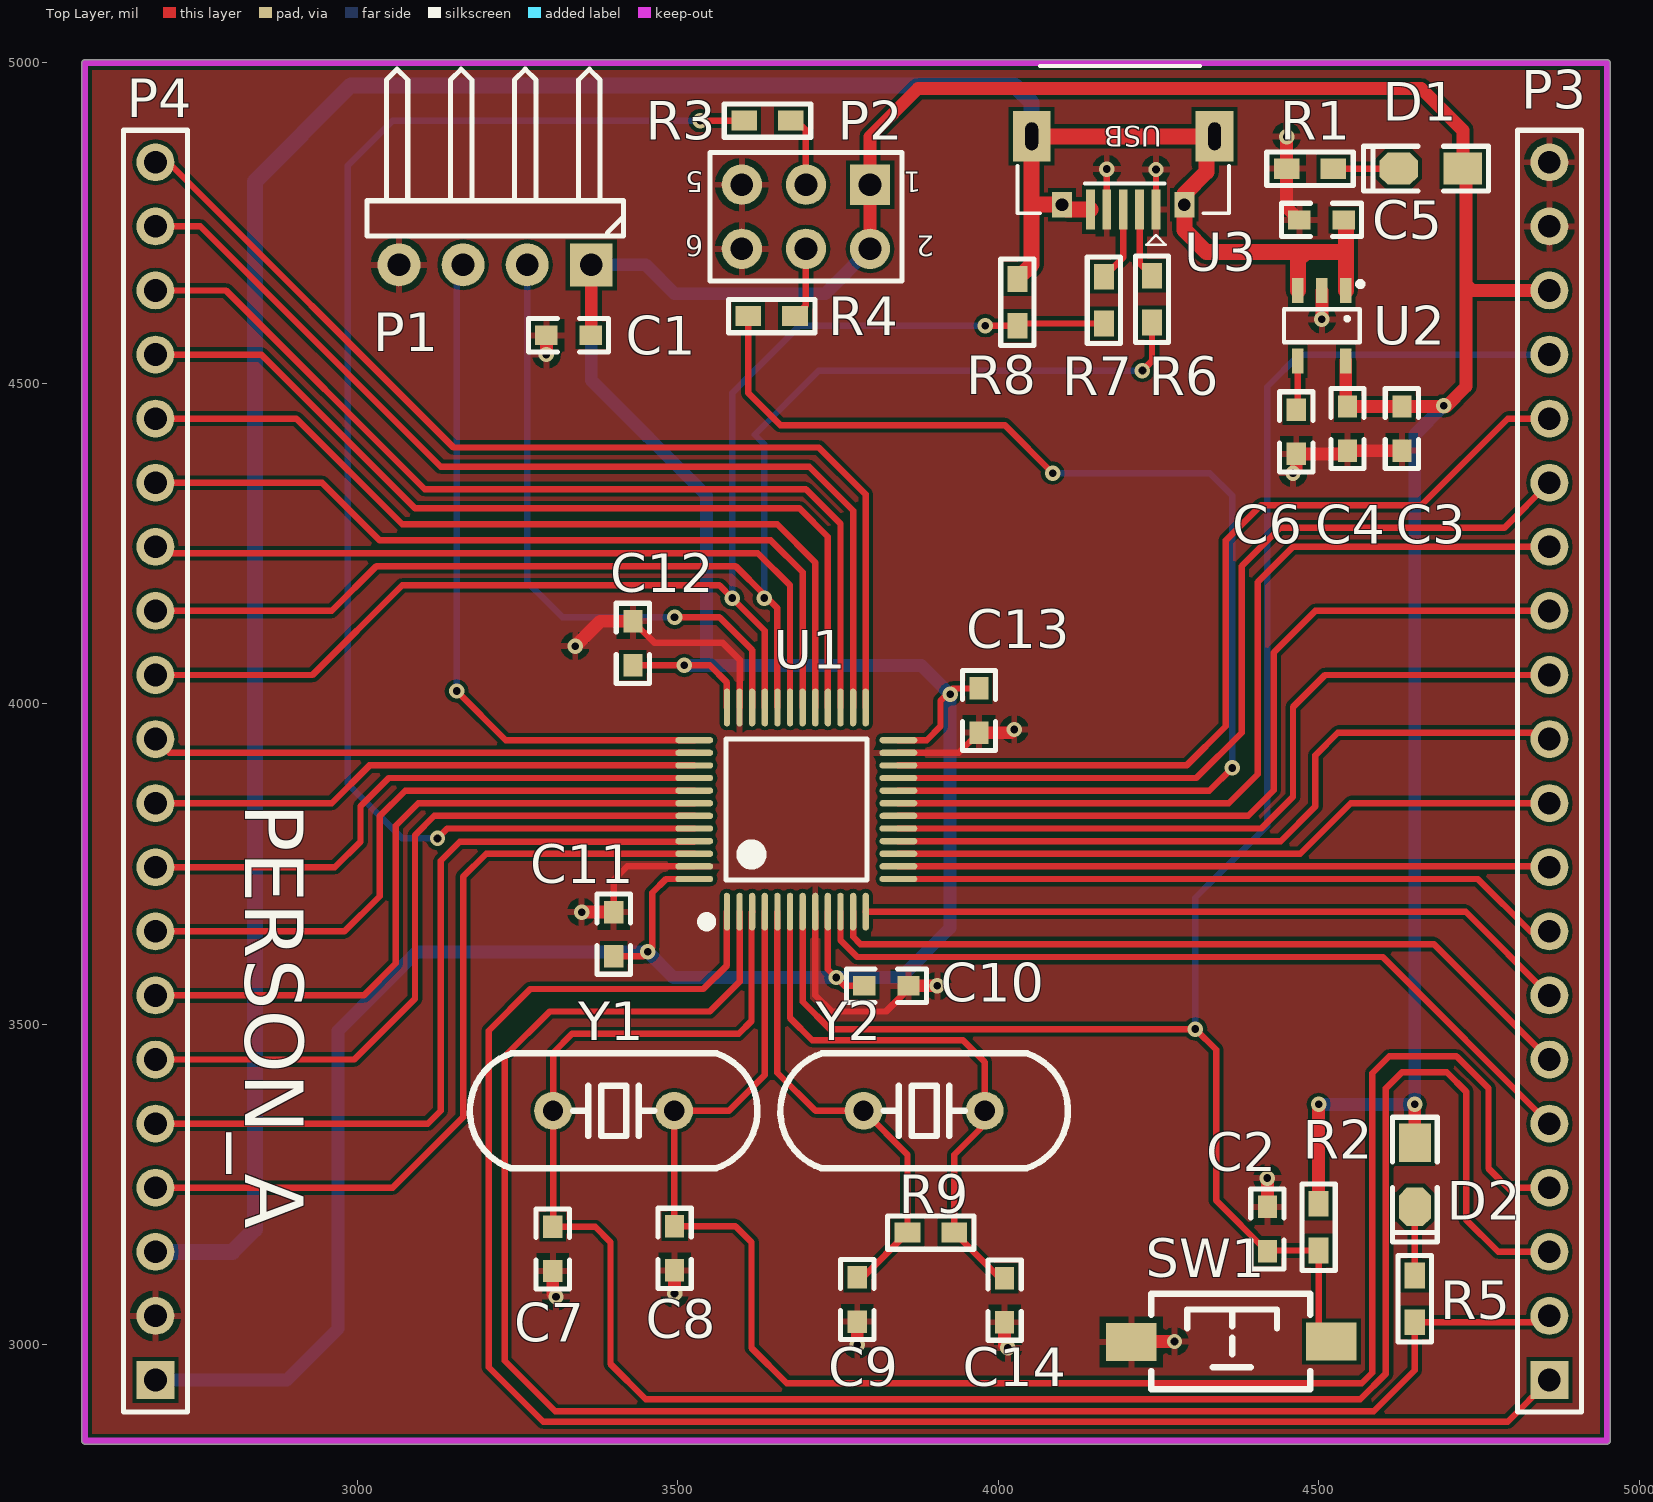
[diagram p0: Top Layer view]
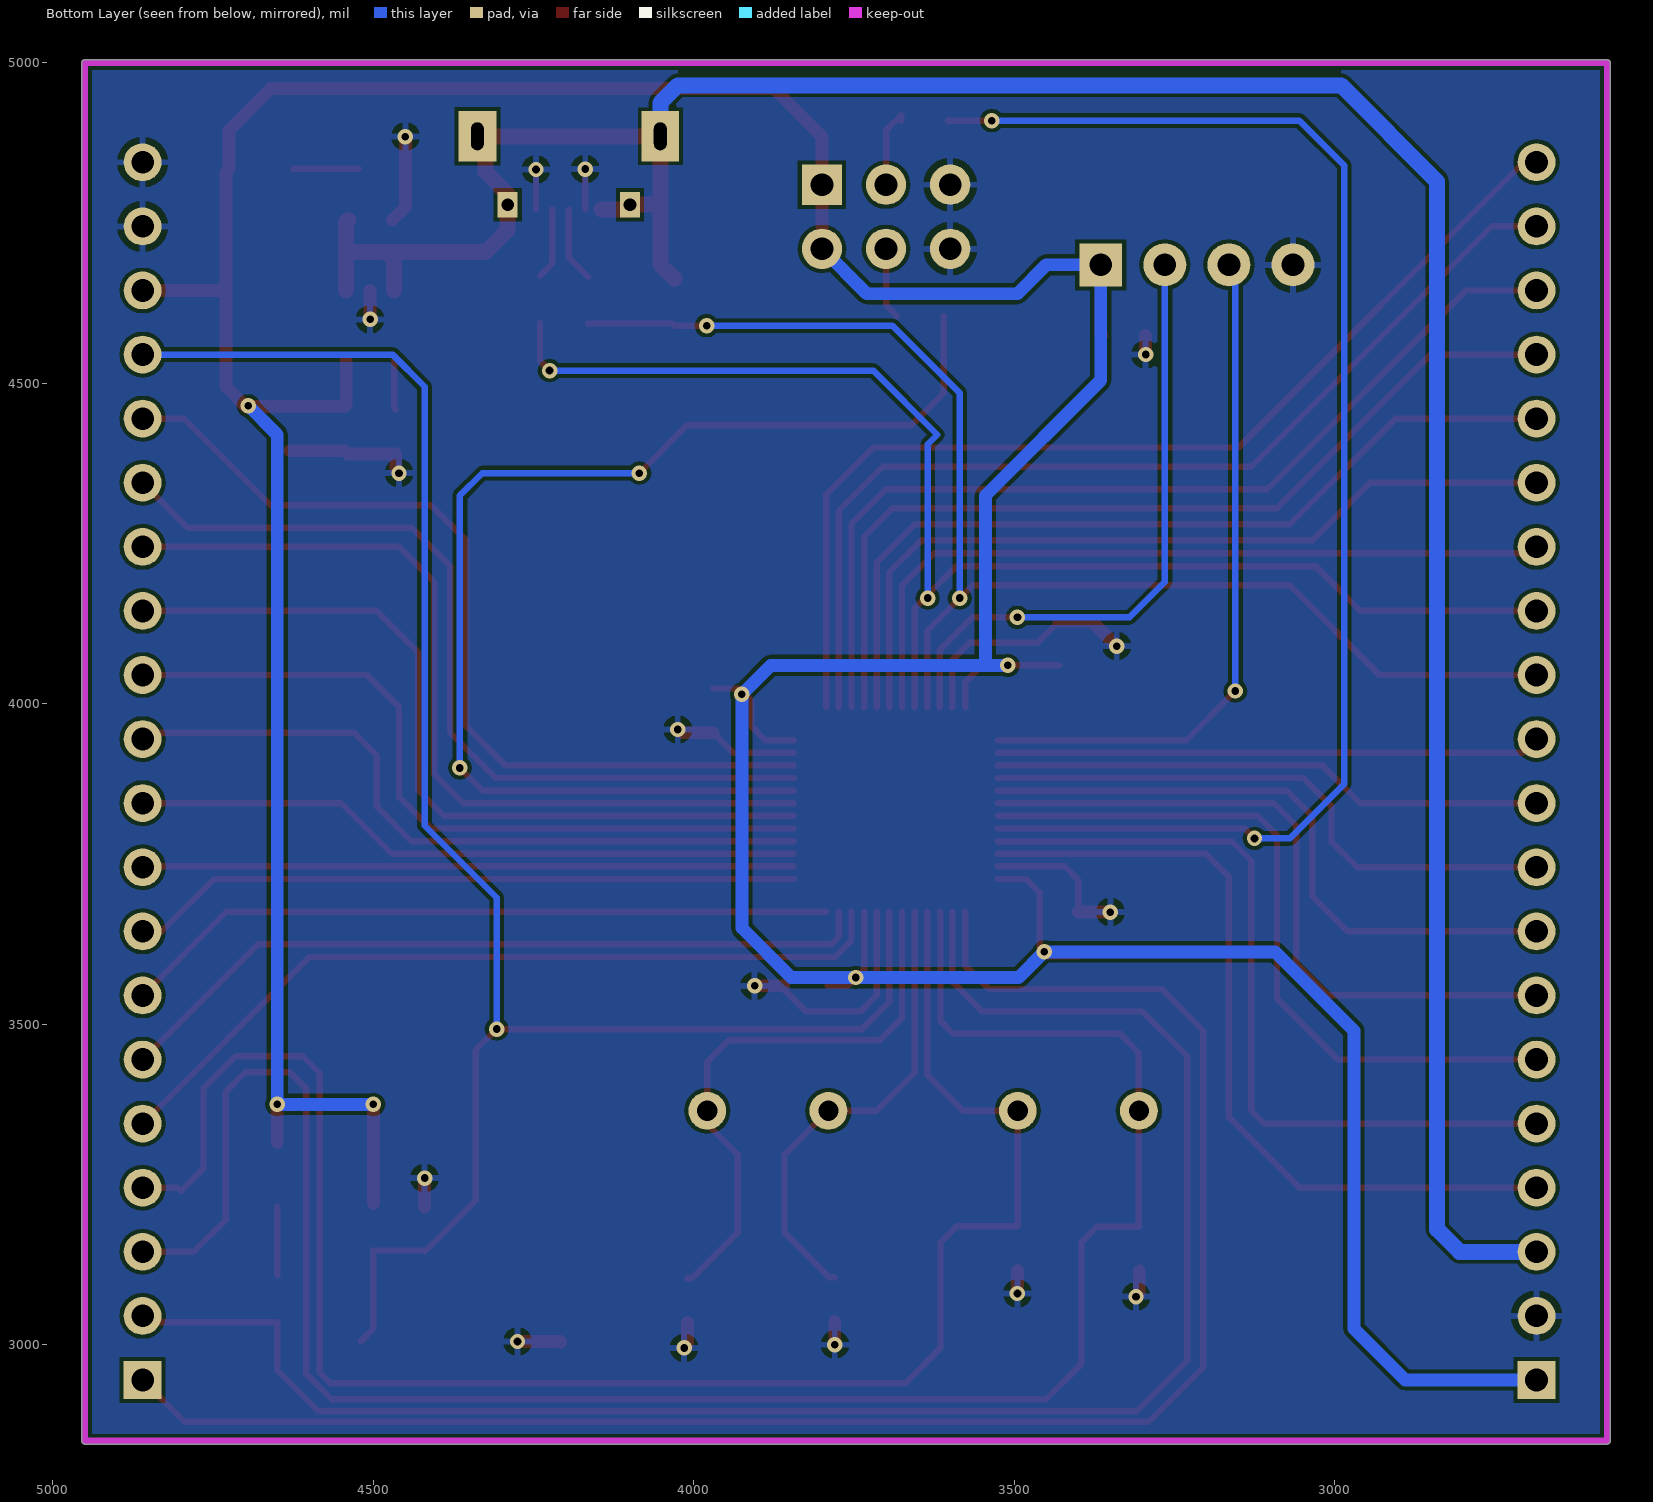
[diagram p1: Bottom Layer view, seen from below]
# Altium PCB MISC82227.PcbDoc
Units mil, origin at the board's own origin, x right, y up, seen from the top; angles counter-clockwise.
Board outline 2385.03 x 2160.03 mil, 2 copper layers (Top Layer, Bottom Layer); 35 components, 50 nets, 168 pads, 34 vias.

## Layer stack, top to bottom (the 12.6 mil dielectric is the usual default, probably not edited)
Top Solder: solder mask 0.4, Solder Resist, Dk 3.5
Top Layer: signal copper 1.4
Dielectric 1: dielectric 12.6, FR-4, Dk 4.8
Bottom Layer: signal copper 1.4
Bottom Solder: solder mask 0.4, Solder Resist, Dk 3.5

## Board outline
2575,2844.99 cw(c2575,2850) 2569.99,2850 2569.99,5000 cw(c2575,5000) 2575,5005.02 4950,5005.02 cw(c4950,5000) 4955.02,5000 4955.02,2850 cw(c4950,2850) 4950,2844.99

## Design rules (kind name [scope] priority, off if disabled: settings)
Clearance [All] p1: gap=6
MinimumSolderMaskSliver [All] p1: minsoldermaskwidth=0
PolygonConnect [All] p1: connectstyle=Relief reliefconductorwidth=10 reliefentries=4 polygonreliefangle="90 Angle" airgapwidth=10
RoutingVias [All] p1: holewidth=28 width=50 viastyle="Through Hole" minholewidth=28 minwidth=50 maxholewidth=28 maxwidth=50
SilkToSilkClearance [All] p1: silktosilkclearance=0
SilkToSolderMaskClearance [IsPad] p1: minsilkscreentomaskgap=0 clearancetoexposedcopper=TRUE
SolderMaskExpansion [All] p1: expansion=4
Width [All] p1: maxlimit=30 minlimit=10 preferedwidth=10
27 further rules are at their usual default settings.

## Components (designator, comment, footprint, x,y, rotation, side; value= is the part's Value field where it differs from the comment)
C1 "105 C0603" "C 0603" 3330,4575 r0 top
C2 "105 C0603" "C 0603" 4420,3180 r270 top
C3 "105 C0603" "C 0603" 4630,4430 r90 top
C4 "105 C0603" "C 0603" 4545,4430 r90 top
C5 "105 C0603" "C 0603" 4505,4755 r0 top
C6 "105 C0603" "C 0603" 4465,4425 r90 top
C7 "22P,0603" "C 0603" 3305,3149 r270 top
C8 "22P,0603" "C 0603" 3495,3150 r270 top
C9 "22P,0603" "C 0603" 3780,3070 r270 top
C10 "105 C0603" "C 0603" 3825,3560 r180 top
C11 "105 C0603" "C 0603" 3400,3640 r270 top
C12 "105 C0603" "C 0603" 3430,4094 r270 top
C13 "105 C0603" "C 0603" 3970,3990 r90 top
C14 "22P,0603" "C 0603" 4010,3069 r270 top
D1 "LED" "LED 0805G" 4675,4835 r180 top
D2 "LED" "LED 0805G" 4650,3265 r270 top
P1 "SWD" HDR-1X4_H 3365,4685 r180 top
P2 "Header 3X2" HDR-3X2 3800,4810 r180 top
P3 "Header 20" HDR1X20 4860,2945 r90 top
P4 "Header 20" HDR1X20 2685,2945 r90 top
R1 "10K R0603" "R 0603" 4486.5,4835 r180 top
R2 "10K R0603" "R 0603" 4500,3183.5 r90 top
R3 "10K R0603" "R 0603" 3640,4910 r0 top
R4 "10K R0603" "R 0603" 3646.5,4605 r180 top
R5 "10K R0603" "R 0603" 4650,3071.5 r270 top
R6 "20R,0603" "R 0603" 4240,4631.5 r270 top
R7 "20R0603" "R 0603" 4165,4630 r270 top
R8 "4.7K,0603" "R 0603" 4030,4626.5 r270 top
R9 "1M0603" "R 0603" 3895,3175 r180 top
SW1 "SW-PB_V" "TSW SMD-3*6*2.5" 4365,3005 r0 top
U1 "stm32f103c8t6_48pin" "TQFP48 7x7_L" 3685,3835 r0 top
U2 "RT9193" SOT23-5L 4505,4590 r180 top
U3 "USB-mrico" USB-micro_B 4195,4885.51 r180 top
Y1 "32.768K" "XTAL-49S DIP" 3400,3365 r180 top
Y2 "8M" "XTAL-49S DIP" 3884.49,3365 r180 top

## Footprints (in the part's own frame and the unit in brackets; to place one, negate y for a bottom-side part, rotate by r counter-clockwise, add the part's x,y. Pads: shape width x height; smd on the part's side, far side on the other; paste and mask are expansions set on the pad)
"C 0603" [mil] "无极性贴片电容"
  rect 35x30 smd: 1(-35,0) 2(34,0)
  silkscreen extent -63,-26 62,26, body extent -31,-16 31,16, height 32
HDR1X20 [mm] "Connector; Header; 20 Position"
  rect 1.5x1.5 hole 0.9: 1(0,0)
  round 1.5 hole 0.9: 2(2.54,0) 3(5.08,0) 4(7.62,0) 5(10.16,0) 6(12.7,0) 7(15.24,0) 8(17.78,0) 9(20.32,0) 10(22.86,0) 11(25.4,0) 12(27.94,0) 13(30.48,0) 14(33.02,0) 15(35.56,0) 16(38.1,0) 17(40.64,0) 18(43.18,0) 19(45.72,0) 20(48.26,0)
  silkscreen extent -1.27,-1.27 49.53,1.27
HDR-1X4_H [mm] "弯脚排针，4脚"
  rect 1.7x1.7 hole 0.9: 1(0,0)
  round 1.7 hole 0.9: 2(2.54,0) 3(5.08,0) 4(7.62,0)
  silkscreen extent -1.27,-7.76 8.89,-1.14, body extent -1.27,-7.77 8.89,1.27, height 4.85
HDR-3X2 [mm] "双排排针，3x2脚"
  rect 1.6x1.6 hole 0.9: 1(0,0)
  round 1.6 hole 0.9: 2(0,2.54) 3(2.54,0) 4(2.54,2.54) 5(5.08,0) 6(5.08,2.54)
  silkscreen extent -1.27,-1.27 6.35,3.81, body extent -1.27,-1.27 6.35,3.81, height 8.5
"LED 0805G" [mil] "绿色0805LED"
  rect 60x50 smd: 1(-50,0)
  oct 60x50 smd: 2(50,0)
  silkscreen extent -90,-35 105,35, body extent -39,-25 39,25, height 32
"R 0603" [mil] "1/10W贴片电阻"
  rect 40x31.5 smd: 1(-36.5,0) 2(36.5,0)
  silkscreen extent -68,-26 68,26, body extent -31,-16 31,16, height 16
SOT23-5L [mm] "3x1.6x1.1mm(长宽高)"
  rect 0.45x1 smd: 1(-0.95,-1.4) 2(0,-1.4) 3(0.95,-1.4) 4(0.95,1.4) 5(-0.95,1.4)
  silkscreen extent -1.6,-1.73 1.5,0.66, body extent -1.5,-1.4 1.5,1.4, height 1.15
"TQFP48 7x7_L" [mm] "48脚，体宽：7x7mm, 脚距：0.5mm"
  oval 0.25x1.5 smd: 1(-2.75,-4.046) 2(-2.25,-4.046) 3(-1.75,-4.046) 4(-1.25,-4.046) 5(-0.75,-4.046) 6(-0.25,-4.046) 7(0.25,-4.046) 8(0.75,-4.046) 9(1.25,-4.046) 10(1.75,-4.046) 11(2.25,-4.046) 12(2.75,-4.046) 25(2.75,4.046) 26(2.25,4.046) 27(1.75,4.046) 28(1.25,4.046) 29(0.75,4.046) 30(0.25,4.046) 31(-0.25,4.046) 32(-0.75,4.046) 33(-1.25,4.046) 34(-1.75,4.046) 35(-2.25,4.046) 36(-2.75,4.046)
  oval 1.5x0.25 smd: 13(4.046,-2.75) 14(4.046,-2.25) 15(4.046,-1.75) 16(4.046,-1.25) 17(4.046,-0.75) 18(4.046,-0.25) 19(4.046,0.25) 20(4.046,0.75) 21(4.046,1.25) 22(4.046,1.75) 23(4.046,2.25) 24(4.046,2.75) 37(-4.046,2.75) 38(-4.046,2.25) 39(-4.046,1.75) 40(-4.046,1.25) 41(-4.046,0.75) 42(-4.046,0.25) 43(-4.046,-0.25) 44(-4.046,-0.75) 45(-4.046,-1.25) 46(-4.046,-1.75) 47(-4.046,-2.25) 48(-4.046,-2.75)
  silkscreen extent -3.68,-4.57 2.79,2.79, body extent -4.5,-4.5 4.5,4.5, height 1.05
"TSW SMD-3*6*2.5" [mm] "3*6*2.5mm"
  rect 2x1.5 smd: 1(-3.996,-0.02) 2(3.937,0)
  silkscreen extent -3.21,-1.9 3.09,1.9, body extent -4,-1.88 4,1.62, height 2.59
USB-micro_B [mm] "micro型USB ，5.7*7.8*2.5mm"
  rect 0.35x1.6 smd: 1(-1.3,2.9) 2(-0.65,2.9) 3(0,2.9) 4(0.65,2.9) 5(1.3,2.9)
  rect 1.5x2 hole 0.5 slot 1.1 at 90 deg: 5(-3.625,0) 5(3.625,0)
  rect 0.8x1 hole 0.5: 5(-2.425,2.71) 5(2.425,2.71)
  silkscreen extent -4.19,-2.79 4.19,4.3, body extent -4,-2.71 4,2.89, height 2.8
"XTAL-49S DIP" [mm]
  round 1.5 hole 0.8: 1(-2.4,0) 2(2.4,0)
  silkscreen extent -5.7,-2.28 5.7,2.28, body extent -5.68,-2.35 5.68,2.3, height 3.5

## Part data
C1 C2 C3 C4 C5 C6 C10 C11 C12 C13: library part Cap
C7 C8 C9 C14: library part Cap, "Capacitor"
P1: library part "Header 4", "Header, 4-Pin"
P2: "Header, 3-Pin, Dual row"
P3 P4: "Header, 20-Pin"
R1 R2 R3 R4 R5: library part Res2
R6 R7 R8 R9: library part Res2, "Resistor"
U2: library part RT9193X_5P
U3: library part usb-STM
Y1 Y2: library part XTAL, "Crystal Oscillator"

## Via types
v1: diameter 24, hole 12, Top Layer to Bottom Layer, 34 vias

## Nets (pads, with @x,y where several pads share a name; then routed paths per layer and width w, separated by ;. In a path a pad name is that pad's centre, name@x,y a point inside that pad or via, vN(x,y) a via of type N, cw(c..) or ccw(c..) an arc to the next point about the centre after c; other vN are vias at no path point)
5V: C5.2 P4.3 R8.1 U2.1 U2.3 U3.5 | length 4362.8
  Top Layer w25: R8.1 4052.28,4685.28 4052.28,4780 ; U3.5@4143.82,4771.34 4107.01,4771.34 4099.53,4778.82 4053.46,4778.82 4052.28,4780 ; U2.3 4467.6,4692.6 4480,4705 ; C5.2 4542.4,4751.6 4542.4,4705 ; U2.1 4542.4,4705 ; 4052.28,4780 4052.28,4885.51 4337.72,4885.51 4325,4872.8 4325,4830 4290.47,4795.47 4290.47,4778.82 4290.47,4739.53 4325,4705 4480,4705 ; 4480,4705 4542.4,4705
  Bottom Layer w25: P4.3 2805,3145 2840,3180 2840,4815 2990,4965 4025,4965 4052.28,4937.72 U3.5@4052.28,4885.51
BOOT0: R3.1 U1.44 | length 2194.8
  Top Layer w10: v1(3125,3790) 3140.47,3805.47 U1.44 ; v1(3535,4910) R3.1
  Bottom Layer w10: v1(3125,3790) 3070,3790 2985,3875 2985,4840 3055,4910 v1(3535,4910)
BOOT1: R4.2 U1.20 | length 1901.7
  Top Layer w10: R4.2 3610,4485 3660,4435 4010,4435 v1(4085,4360) ; U1.20 4329.53,3864.53 v1(4365,3900)
  Bottom Layer w10: v1(4085,4360) 4330,4360 4365,4325 v1(4365,3900)
GND: C1.1 C2.1 C3.1 C4.1 C5.1 C6.1 C7.2 C8.2 C9.2 C10.1 C11.1 C12.1 C13.1 C14.2 P1.4 P2.5 P2.6 P3.19 P3.20 P4.2 R1.2 SW1.1 U1.8 U1.23 U1.35 U1.47 U2.2 U3.1 U3.4 | length 1962.4
  Top Layer w10: C11.1 3400,3725 3421.42,3746.42 U1.47 ; C12.1 3464,4095 3570,4095 3596.42,4068.58 U1.35 ; U1.8 3714.53,3545.47 3740,3520 3825,3520 3860,3555 C10.1 ; U1.23 3938.58,3923.58 C13.1 ; U3.4 v1(4169.41,4834.41) v1@4170,4835 ; v1@4245,4835 v1(4246.18,4833.82) U3.1
  Top Layer w20: v1(3295,4545) C1.1 ; C7.2 3305,3080 v1(3310,3075) ; v1(3340,4090) 3379,4129 C12.1 ; v1(3350,3675) C11.1 ; v1(3495,3080) C8.2 ; v1(3780,3000) C9.2 ; C10.1 v1(3905,3560) ; C13.1 4020,3955 v1(4025,3960) ; C14.2 4010,3000 v1(4015,2995) ; SW1.1 4208.47,3005 v1(4275,3005) ; C2.1 v1(4420,3260) ; v1(4450,4885) R1.2 4450,4775 C5.1 ; v1(4460,4360) 4465,4365 C6.1 4540,4390 C4.1 C3.1 ; v1(4505,4600) U2.2
NetC6_2: C6.2 U2.4 | length 77
  Top Layer w10: C6.2 4467.6,4461.6 U2.4
NetD1_2: D1.2 R1.1 | length 102
  Top Layer w10: R1.1 D1.2
NetD2_2: D2.2 R5.1 | length 107
  Top Layer w10: R5.1 D2.2
NetP2_3: P2.3 R3.2 | length 126.7
  Top Layer w10: R3.2 3676.5,4918.5 3700,4895 P2.3
NetP2_4: P2.4 R4.1 | length 112
  Top Layer w10: R4.1 3700,4622 P2.4
NetR6_1: R6.1 U3.2 | length 111.4
  Top Layer w10: U3.2 4220.59,4687.41 R6.1
NetR7_1: R7.1 U3.3 | length 117.3
  Top Layer w10: R7.1 4195,4696.5 U3.3
OSCIN: C9.1 R9.2 U1.5 Y2.2 | length 736.2
  Top Layer w10: U1.5 3655.47,3424.53 3715,3365 Y2.2 3858.5,3296.5 R9.2 3788.5,3105 C9.1
OSCOUT: C14.1 R9.1 U1.6 Y2.1 | length 891.8
  Top Layer w10: U1.6 3675.16,3509.84 3710,3475 3945,3475 3978.98,3441.02 Y2.1 3978.98,3343.98 3931.5,3296.5 R9.1 4002.5,3104 C14.1
PA0: P3.5 U1.10 | length 1269.2
  Top Layer w10: U1.10 3753.9,3631.1 3780,3605 4600,3605 P3.5
PA1: P3.6 U1.11 | length 1205
  Top Layer w10: U1.11 3773.58,3636.42 3785,3625 4680,3625 P3.6
PA2: P3.7 U1.12 | length 1120.9
  Top Layer w10: U1.12 4729.29,3675.71 P3.7
PA3: P3.8 U1.13 | length 1049.6
  Top Layer w10: U1.13 4748.27,3726.73 4830,3645 P3.8
PA4: P3.9 U1.14 | length 1016.3
  Top Layer w10: U1.14 4858.58,3746.42 P3.9
PA5: P3.10 U1.15 | length 1048.4
  Top Layer w10: U1.15 4471.1,3766.1 4550,3845 P3.10
PA6: P3.11 U1.16 | length 1136.8
  Top Layer w10: U1.16 4440.79,3785.79 4495,3840 4495,3920 4530,3955 4850,3955 P3.11
PA7: P3.12 U1.17 | length 1196.9
  Top Layer w10: U1.17 4410.47,3805.47 4460,3855 4460,3995 4510,4045 P3.12
PA8: P4.16 U1.29 | length 1348.7
  Top Layer w10: P4.16 2905,4445 3070,4280 3655,4280 3714.53,4220.47 U1.29
PA9: P4.15 U1.30 | length 1278.6
  Top Layer w10: P4.15 2945,4345 3035,4255 3645,4255 3694.84,4205.16 U1.30
PA10: P4.14 U1.31 | length 1205.6
  Top Layer w10: P4.14 2695,4235 3625,4235 3675.16,4184.84 U1.31
PA11: P4.13 R6.2 U1.32 | length 2173.6
  Top Layer w10: P4.13 2960,4145 3030,4215 3590,4215 3635,4170 v1(3635,4165) 3640,4165 3655.47,4149.53 U1.32 ; v1(4225,4520) 4240,4535 R6.2
  Bottom Layer w10: v1(3635,4165) 3635,4405 3620,4420 3720,4520 v1(4225,4520)
PA12: P4.12 R7.2 R8.2 U1.33 | length 2103
  Top Layer w10: P4.12 2930,4045 3070,4185 3565,4185 v1(3585,4165) 3635.79,4114.21 U1.33 ; v1(3980,4590) R8.2 4033.5,4593.5 R7.2
  Bottom Layer w10: v1(3585,4165) 3585,4485 3690,4590 v1(3980,4590)
PA15: P4.11 U1.38 | length 849.6
  Top Layer w10: P4.11 2706.42,3923.58 U1.38
PB0: P3.13 U1.18 | length 1274.1
  Top Layer w10: U1.18 4390.16,3825.16 4430,3865 4430,4080 4495,4145 P3.13
PB1: P3.14 U1.19 | length 1357.2
  Top Layer w10: U1.19 4359.84,3844.84 4405,3890 4405,4190 4460,4245 P3.14
PB3: P4.10 U1.39 | length 865.1
  Top Layer w10: P4.10 2960,3845 3018.9,3903.9 U1.39
PB4: P4.9 U1.40 | length 930.6
  Top Layer w10: P4.9 2965,3745 3005,3785 3005,3840 3049.21,3884.21 U1.40
PB5: P4.8 U1.41 | length 1004.9
  Top Layer w10: P4.8 2980,3645 3035,3700 3035,3825 3074.53,3864.53 U1.41
PB6: P4.7 U1.42 | length 1091
  Top Layer w10: P4.7 3010,3545 3060,3595 3060,3810 3095,3845 3095.16,3844.84 U1.42
PB7: P4.6 U1.43 | length 1147.6
  Top Layer w10: P4.6 2995,3445 3090,3540 3090,3795 3120.16,3825.16 U1.43
PB8: P4.5 U1.45 | length 1251.7
  Top Layer w10: P4.5 3110,3345 3130,3365 3130,3755 3160,3785 3524.92,3785 U1.45
PB9: P4.4 U1.46 | length 1276.2
  Top Layer w10: P4.4 3055,3245 3165,3355 3165,3730 3201.1,3766.1 U1.46
PB10: P3.15 U1.21 | length 1358.9
  Top Layer w10: U1.21 4309.21,3884.21 4380,3955 4380,4215 4440,4275 4790,4275 P3.15
PB11: P3.16 U1.22 | length 1409.7
  Top Layer w10: U1.22 4293.9,3903.9 4355,3965 4355,4255 4410,4310 4660,4310 4795,4445 P3.16
PB12: P4.20 U1.25 | length 1655.4
  Top Layer w10: P4.20 2705,4845 3150,4400 3720,4400 3793.27,4326.73 U1.25
PB13: P4.19 U1.26 | length 1579.4
  Top Layer w10: P4.19 2755,4745 3130,4370 3705,4370 3773.58,4301.42 U1.26
PB14: P4.18 U1.27 | length 1506.4
  Top Layer w10: P4.18 2795,4645 3105,4335 3700,4335 3753.9,4281.1 U1.27
PB15: P4.17 U1.28 | length 1433.4
  Top Layer w10: P4.17 2850,4545 3090,4305 3690,4305 3734.21,4260.79 U1.28
PC13: P3.2 R5.2 U1.2 | length 2767.3
  Top Layer w10: U1.2 3596.42,3566.42 3550,3520 3300,3520 3230,3450 3230,2975 3309,2896 4586,2896 4650,2960 R5.2 4850,3035 P3.2
PC14: C7.1 P3.3 U1.3 Y1.2 | length 3255.7
  Top Layer w10: U1.3 3615,3674.61 3615,3505 3595,3485 3335,3485 3305.51,3455.51 Y1.2 3305.51,3184.51 C7.1 3371,3184 3395,3160 3395,2970 3450,2915 4565,2915 4605,2955 4605,3400 4630,3425 4700,3425 4730,3395 4730,3195 4780,3145 P3.3
PC15: C8.1 P3.4 U1.4 Y1.1 | length 2810
  Top Layer w10: U1.4 3635.79,3420.79 3580,3365 Y1.1 3494.49,3185.51 C8.1 3590,3185 3615,3160 3615,2995 3670,2940 4567.37,2940 4583.69,2956.31 4583.69,3423.69 4610,3450 4715,3450 4765,3400 4765,3275 4800,3240 4805,3245 P3.4
RESET: C2.2 P3.17 R2.1 SW1.2 U1.7 | length 2905.1
  Top Layer w10: U1.7 3694.84,3535.16 3737.5,3492.5 v1(4307.5,3492.5) 4340,3460 4340,3225 4419,3146 C2.2 4421,3147 R2.1 4500,3025 SW1.2
  Bottom Layer w10: v1(4307.5,3492.5) 4307.5,3697.5 4420,3810 4420,4495 4470,4545 P3.17
SWDCLK: P1.3 U1.37 | length 1071.6
  Top Layer w10: v1(3155,4020) 3231.73,3943.27 U1.37
  Bottom Layer w10: v1(3155,4020) 3155,4675 P1.3
SWDIO: P1.2 U1.34 | length 979.7
  Top Layer w10: v1(3495,4135) 3565,4135 3616.1,4083.9 U1.34
  Bottom Layer w10: P1.2 3265,4190 3320,4135 v1(3495,4135)
VBAT: P3.1 U1.1 | length 2740
  Top Layer w10: U1.1 3576.73,3591.73 3540,3555 3270,3555 3205,3490 3205,2965 3290,2880 4795,2880 P3.1
VCC3V3: C1.2 C3.2 C4.2 C10.2 C11.2 C12.2 C13.2 D1.1 D2.1 P1.1 P2.1 P2.2 P3.18 P4.1 R2.2 U1.9 U1.24 U1.36 U1.48 U2.5 | length 8128.8
  Top Layer w10: C11.2 3446,3606 v1(3453,3613) 3460,3620 3460,3705 3481.73,3726.73 U1.48 ; C12.2 v1(3510,4060) 3550,4060 3576.73,4033.27 U1.36 ; U1.9 3734.21,3585.79 v1(3747.11,3572.89) 3760,3560 C10.2 ; U1.24 3888.27,3943.27 3910,3965 3910,4005 3929,4024 C13.2
  Top Layer w20: C1.2 3365,4576 P1.1 ; P2.2 P2.1 3800,4885 3875,4960 4660,4960 4725,4895 D1.1 4730,4830 4730,4655 ; R2.2 v1(4500,3375) ; U2.5 4542.4,4466.6 C4.2 C3.2 4699,4464 4730,4495 4730,4655 ; D2.1 v1(4650,3375) ; P3.18 4740,4645 4730,4655
  Bottom Layer w20: P4.1 2890,2945 2970,3025 2970,3490 3093,3613 v1(3453,3613) 3493.11,3572.89 v1(3747.11,3572.89) 3847.89,3572.89 3925,3650 v1(3925,4015) 3880,4060 3545,4060 ; v1(3510,4060) 3545,4060 ; P2.2 3730,4640 3495,4640 3450,4685 P1.1 3365,4505 3545,4325 3545,4060 ; v1(4500,3375) v1(4650,3375) 4650,4420 v1(4695,4465)

## Polygon pours and split planes (outlines as drawn)
GND on Top Layer "D" (solid, remove dead copper, pour order 0): 1940,5325 1990,5275 5545,5275 5545,2815 5295,2565 5120,2740 2080,2740
GND on Bottom Layer "D" (solid, remove dead copper, pour order 2): 1980,5270 5640,5270 5645,5265 5525,5145 5525,2530 1825,2530 1765,2470

## Keep-outs
Keep-Out Layer:
  lines w10: 2620,5000 4950,5000 4950,4860 4950,2850 2575,2850 2575,5000 2635,5000

## Silkscreen, mask and mechanical layers (free items; w line width, h text height)
Top Overlay:
  text "PERSON_A" at 2795,3845 h157.48 r270